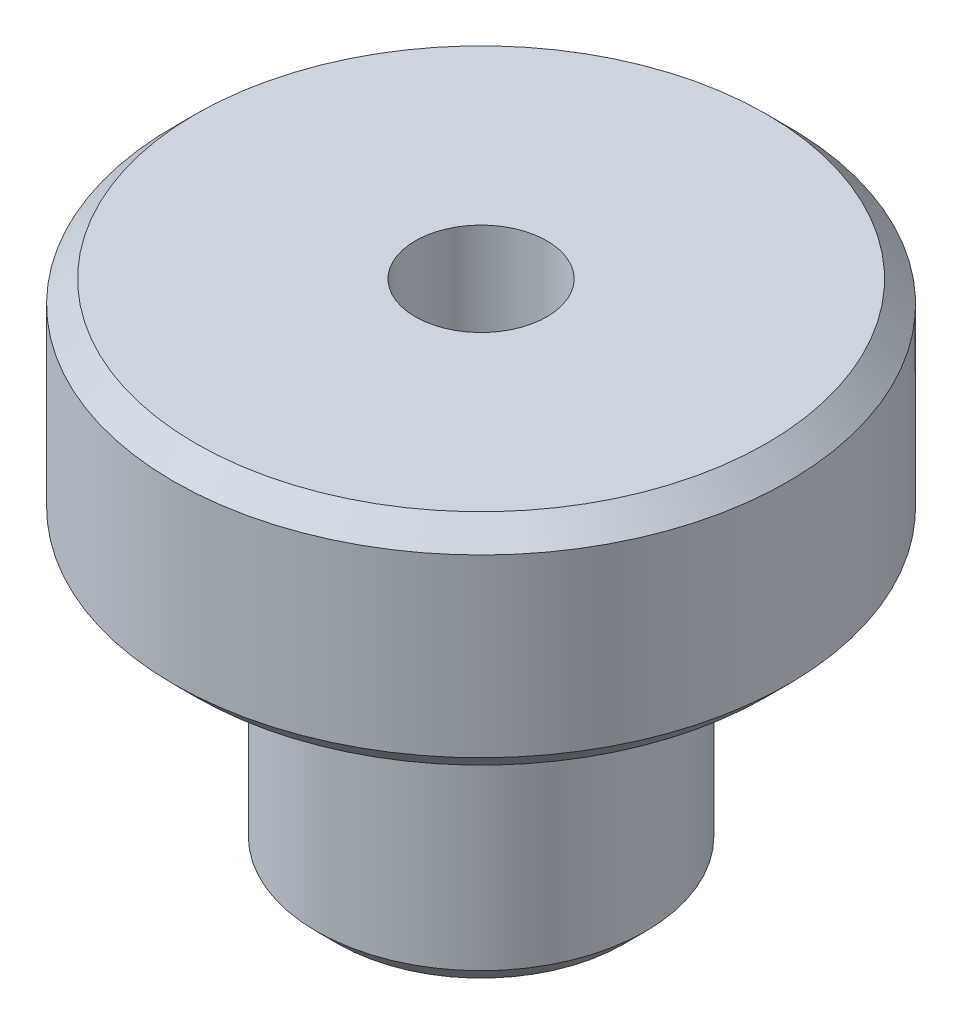
from build123d import *

# Parameters (mm, degrees)
SKETCH1_R           = 7.5
SKETCH1_R_2         = 3
BOSS_EXTRUDE1_DEPTH = 23
BOSS_EXTRUDE2_START = -10
SKETCH2_R           = 14
SKETCH2_R_2         = 3
BOSS_EXTRUDE2_DEPTH = 10
CHAMFER1_SIZE       = 1
SKETCH3_R           = 2
CUT_EXTRUDE1_DEPTH  = 15


with BuildPart() as part:
    # Sketch1 → Boss-Extrude1 (new body)
    with BuildSketch(Plane(origin=(0, 0, 0), x_dir=(1, 0, 0), z_dir=(0, 1, 0))):
        with Locations(Location((0, 0, 0), (0, 0, 270))):
            Circle(SKETCH1_R)
        with Locations(Location((0, 0, 0), (0, 0, 270))):
            Circle(SKETCH1_R_2, mode=Mode.SUBTRACT)
    extrude(amount=BOSS_EXTRUDE1_DEPTH)

    # Sketch2 → Boss-Extrude2 (add)
    with BuildSketch(Plane(origin=(0, 23, 0), x_dir=(1, 0, 0), z_dir=(0, 1, 0)).offset(BOSS_EXTRUDE2_START)):
        with Locations(Location((0, 0, 0), (0, 0, 270))):
            Circle(SKETCH2_R)
        with Locations(Location((0, 0, 0), (0, 0, 270))):
            Circle(SKETCH2_R_2, mode=Mode.SUBTRACT)
    extrude(amount=BOSS_EXTRUDE2_DEPTH)

    # Chamfer1
    chamfer1_edges = [part.edges().sort_by_distance(p)[0] for p in [
        (0, 23, -14),
        (0, 13, -14),
        (0, 0, -7.5),
    ]]
    chamfer(chamfer1_edges, length=CHAMFER1_SIZE)

    # Sketch3 → Cut-Extrude1 (cut)
    with BuildSketch(Plane(origin=(0, 0, 0), x_dir=(0, 0, -1), z_dir=(1, 0, 0))):
        with Locations((0, 7.039629159)):
            Circle(SKETCH3_R)
    extrude(amount=-CUT_EXTRUDE1_DEPTH, mode=Mode.SUBTRACT)


solid = part.part
